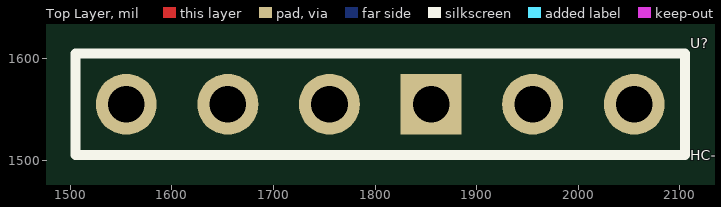
[diagram p0: Top Layer view]
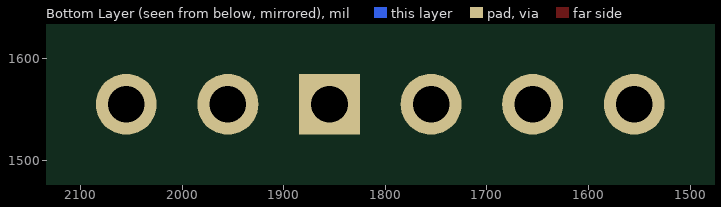
[diagram p1: Bottom Layer view, seen from below]
# Altium PCB MISC84237.PcbDoc
Units mil, origin at the board's own origin, x right, y up, seen from the top; angles counter-clockwise.
Board outline 1635 x 1120 mil, 2 copper layers (Top Layer, Bottom Layer); 1 components, 0 nets, 6 pads, 0 vias.

## Layer stack, top to bottom (the 12.6 mil dielectric is the usual default, probably not edited)
Top Layer: signal copper (thickness not stored)
Dielectric: dielectric 12.6, FR-4, Dk 4.8
Bottom Layer: signal copper (thickness not stored)

## Board outline
2635,1000 1000,1000 1000,2120 2635,2120

## Components (designator, comment, footprint, x,y, rotation, side; value= is the part's Value field where it differs from the comment)
U? "HC-05" HC-05 1805,1555 r0 top

## Footprints (in the part's own frame and the unit in brackets; to place one, negate y for a bottom-side part, rotate by r counter-clockwise, add the part's x,y. Pads: shape width x height; smd on the part's side, far side on the other; paste and mask are expansions set on the pad)
HC-05 [mil]
  round 60 hole 36 paste+4 mask+4: 1(-250,0) 2(-150,0) 3(-50,0) 5(150,0) 6(250,0)
  rect 60x60 hole 36 paste+4 mask+4: 4(50,0)
  silkscreen extent -300,-50 300,50

## Nets (pads, with @x,y where several pads share a name; then routed paths per layer and width w, separated by ;. In a path a pad name is that pad's centre, name@x,y a point inside that pad or via, vN(x,y) a via of type N, cw(c..) or ccw(c..) an arc to the next point about the centre after c; other vN are vias at no path point)
pads on no net: U?.1 U?.2 U?.3 U?.4 U?.5 U?.6

## Silkscreen, mask and mechanical layers (free items; w line width, h text height)
Document:
  lines w0.1: 1817.49,1559.99 1817.51,1560.01